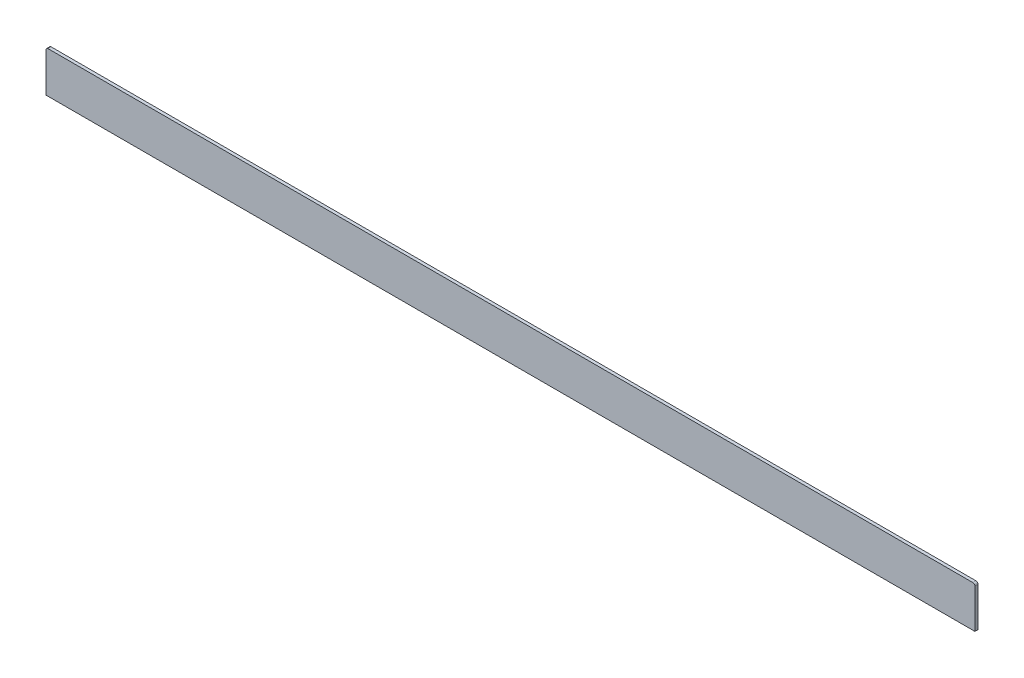
SolidWorks part; units mm, degrees
material "1023 碳钢板 (SS)"
ref_plane "前视基准面" through (0, 0, 0) normal (0, 0, 1) x (1, 0, 0)
ref_plane "上视基准面" through (0, 0, 0) normal (0, 1, 0) x (1, 0, 0)
ref_plane "右视基准面" through (0, 0, 0) normal (1, 0, 0) x (0, 0, -1)
sketch "草图1" plane through (0, 0, 0) normal (0, 0, 1) x (1, 0, 0)
  line L1 (-450, 20) -> (450, 20)
  line L2 (-450, 20) -> (-450, -20)
  line L3 (-450, -20) -> (450, -20)
  line L4 (450, 20) -> (450, -20)
  line L5 (-450, 20) -> (450, -20) construction
  line L6 (-450, -20) -> (450, 20) construction
  point P0 (0, 0)
  dimension "D1" = 900
  dimension "D2" = 40
extrude "凸台-拉伸1" add sketch "草图1" along normal blind 3
fillet "圆角1" radius 2 2 edges at (-450, 20, 1.5) (450, 20, 1.5)
